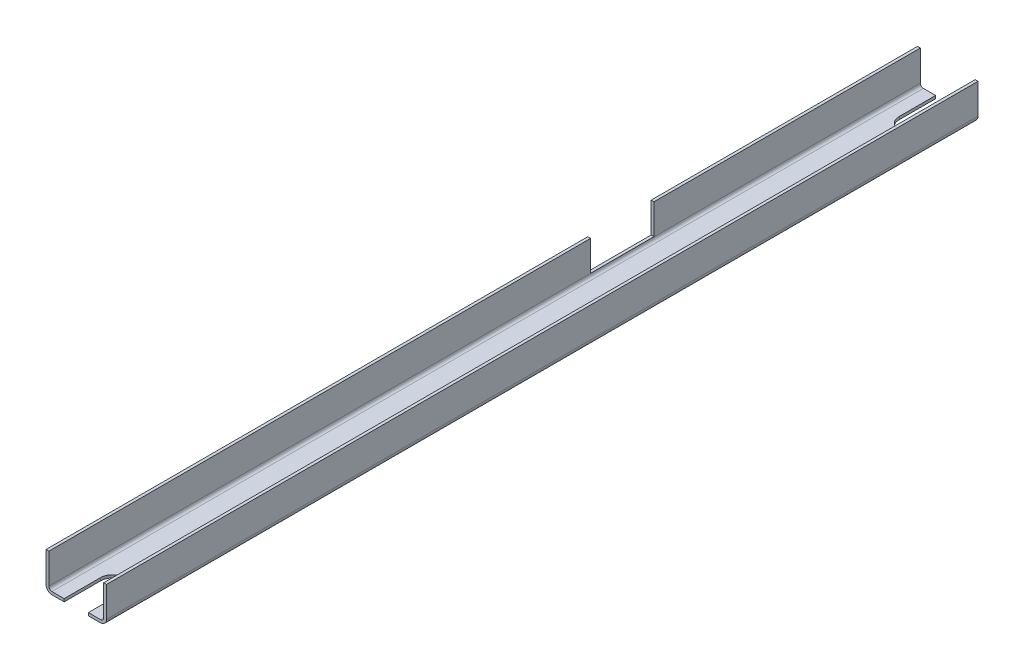
SolidWorks part; units mm, degrees
material "普通碳钢"
ref_plane "Front Plane" through (0, 0, 0) normal (0, 0, 1) x (1, 0, 0)
ref_plane "Top Plane" through (0, 0, 0) normal (0, 1, 0) x (1, 0, 0)
ref_plane "Right Plane" through (0, 0, 0) normal (1, 0, 0) x (0, 0, -1)
sketch "Sketch1" plane through (0, 0, 0) normal (0, 0, 1) x (1, 0, 0)
  line L0 (30.25, 3.1) -> (30.25, 19.05)
  line L1 (3.2, 0) -> (28.55, 0)
  line L2 (0, 3.2) -> (0, 19.05)
  line L3 (3.1, 1.5) -> (28.65, 1.5)
  line L4 (31.75, 3.2) -> (31.75, 19.05)
  line L5 (1.5, 3.1) -> (1.5, 19.05)
  line L6 (1.5, 19.05) -> (0, 19.05)
  line L7 (31.75, 19.05) -> (30.25, 19.05)
  line L8 (1.5, 1.5) -> (30.25, 1.5) construction
  line L9 (1.5, 1.5) -> (1.5, 19.05) construction
  line L10 (30.25, 1.5) -> (30.25, 19.05) construction
  line L11 (31.75, 0) -> (31.75, 19.05) construction
  line L12 (0, 0) -> (31.75, 0) construction
  line L13 (0, 0) -> (0, 19.05) construction
  arc A0 (3.1, 1.5) -> (1.5, 3.1) centre (3.1, 3.1) cw
  arc A1 (28.65, 1.5) -> (30.25, 3.1) centre (28.65, 3.1) ccw
  arc A2 (31.75, 3.2) -> (28.55, 0) centre (28.55, 3.2) cw
  arc A3 (0, 3.2) -> (3.2, 0) centre (3.2, 3.2) ccw
  dimension "D4" = 1.6
  dimension "D5" = 1.6
  dimension "D6" = 3.2
  dimension "D7" = 3.2
  dimension "D2" = 31.75
  dimension "D3" = 1.5
extrude "Boss-Extrude1" add sketch "Sketch1" along normal blind 457.2
sketch "Sketch2" plane through (0, 0, 0) normal (-1, 0, 0) x (0, 0, 1)
  line L0 (139.7, 19.05) -> (139.7, 3.2)
  line L1 (457.2, 19.05) -> (0, 19.05) construction
  line L2 (457.2, 3.2) -> (0, 3.2) construction
  line L3 (172.974, 19.05) -> (172.974, 3.2)
  line L4 (172.974, 3.2) -> (139.7, 3.2)
  line L5 (139.7, 19.05) -> (172.974, 19.05)
  line L6 (0, 19.05) -> (0, 3.2) construction
  dimension "D1" = 139.7
  dimension "D2" = 33.274
extrude "Cut-Extrude1" cut sketch "Sketch2" against normal up to next
sketch "Sketch4" plane through (0, 0, 0) normal (0, -1, 0) x (1, 0, 0)
  line L0 (15.875, 457.2) -> (15.875, 365.102) construction
  line L1 (3.2, 457.2) -> (28.55, 457.2) construction
  line L2 (9.525, 457.2) -> (9.525, 438.15)
  line L3 (22.225, 457.2) -> (22.225, 438.15)
  line L4 (9.525, 457.2) -> (22.225, 457.2)
  arc A0 (9.525, 438.15) -> (22.225, 438.15) centre (15.875, 438.15) ccw
  dimension "D1" = 12.7
  dimension "D2" = 19.05
extrude "Cut-Extrude2" cut sketch "Sketch4" against normal through all
ref_plane "Plane1" through (0, 0, 228.6) normal (0, 0, 1) x (1, 0, 0)
mirror "Mirror1" about plane through (0, 0, 228.6) normal (0, 0, 1) of "Cut-Extrude2"
